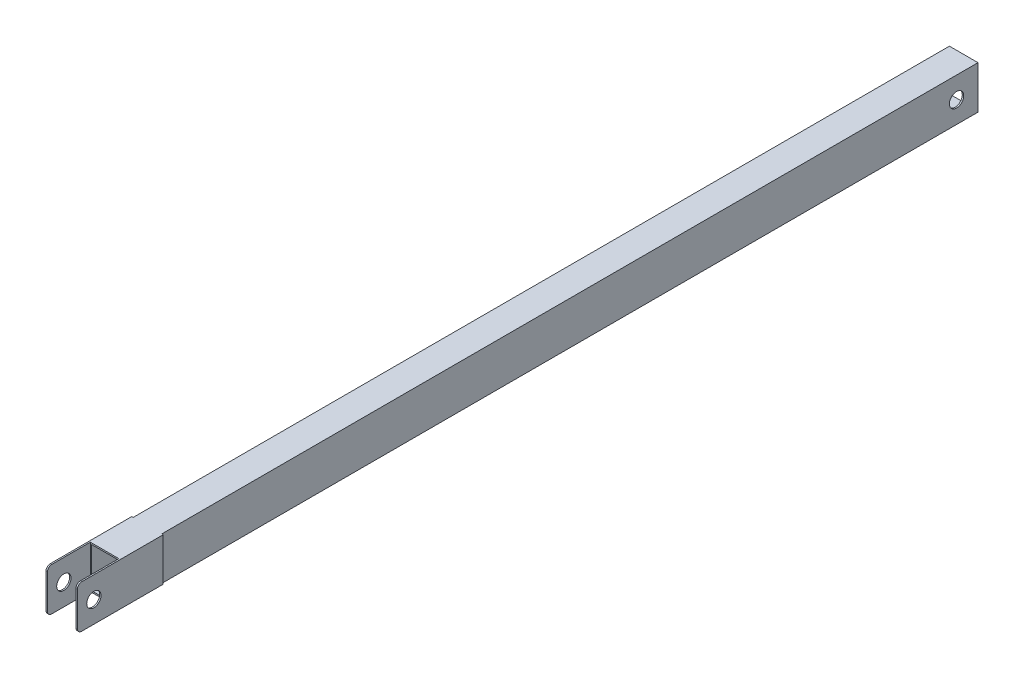
from build123d import *

# Parameters (mm, degrees)
SKETCH1_W           = 20
SKETCH1_H           = 30
SKETCH1_W_2         = 18
SKETCH1_H_2         = 28
BOSS_EXTRUDE1_DEPTH = 601
BOSS_EXTRUDE2_DEPTH = 1
SKETCH4_R           = 5
CUT_EXTRUDE1_DEPTH  = 633.095720599
SKETCH5_R           = 5
CUT_EXTRUDE2_DEPTH  = 633.061705848


with BuildPart() as part:
    # Sketch1 → Boss-Extrude1 (new body)
    with BuildSketch(Plane.XY):
        with Locations((10, -15)):
            Rectangle(SKETCH1_W, SKETCH1_H)
        with Locations((10, -15)):
            Rectangle(SKETCH1_W_2, SKETCH1_H_2, mode=Mode.SUBTRACT)
    extrude(amount=BOSS_EXTRUDE1_DEPTH)

    # Sketch3 → Boss-Extrude2 (add)
    with BuildSketch(Plane.ZY):
        with BuildLine():
            Line((571, -30), (601, -30))
            Line((601, -30), (628, -30))
            ThreePointArc((628, -30), (630.121320344, -29.121320344), (631, -27))
            Line((631, -27), (631, -3))
            ThreePointArc((631, -3), (630.121320344, -0.878679656), (628, 0))
            Line((628, 0), (601, 0))
            Line((601, 0), (571, 0))
            Line((571, 0), (571, -30))
        make_face()
    boss_extrude2 = extrude(amount=BOSS_EXTRUDE2_DEPTH)

    # Mirror2: Boss-Extrude2 across plane
    add(boss_extrude2.mirror(Plane(origin=(10, 0, 0), x_dir=(0, 0, 1), z_dir=(1, 0, 0))))

    # Sketch4 → Cut-Extrude1 (cut, through all)
    with BuildSketch(Plane(origin=(21, 0, 0), x_dir=(0, 0, -1), z_dir=(1, 0, 0))):
        with Locations(Location((-619.5, -15, 0), (0, 0, 90))):
            Circle(SKETCH4_R)
    extrude(amount=-CUT_EXTRUDE1_DEPTH, mode=Mode.SUBTRACT)

    # Sketch5 → Cut-Extrude2 (cut, through all)
    with BuildSketch(Plane.ZY):
        with Locations(Location((15, -15, 0), (0, 0, 270))):
            Circle(SKETCH5_R)
    extrude(amount=-CUT_EXTRUDE2_DEPTH, mode=Mode.SUBTRACT)


solid = part.part
